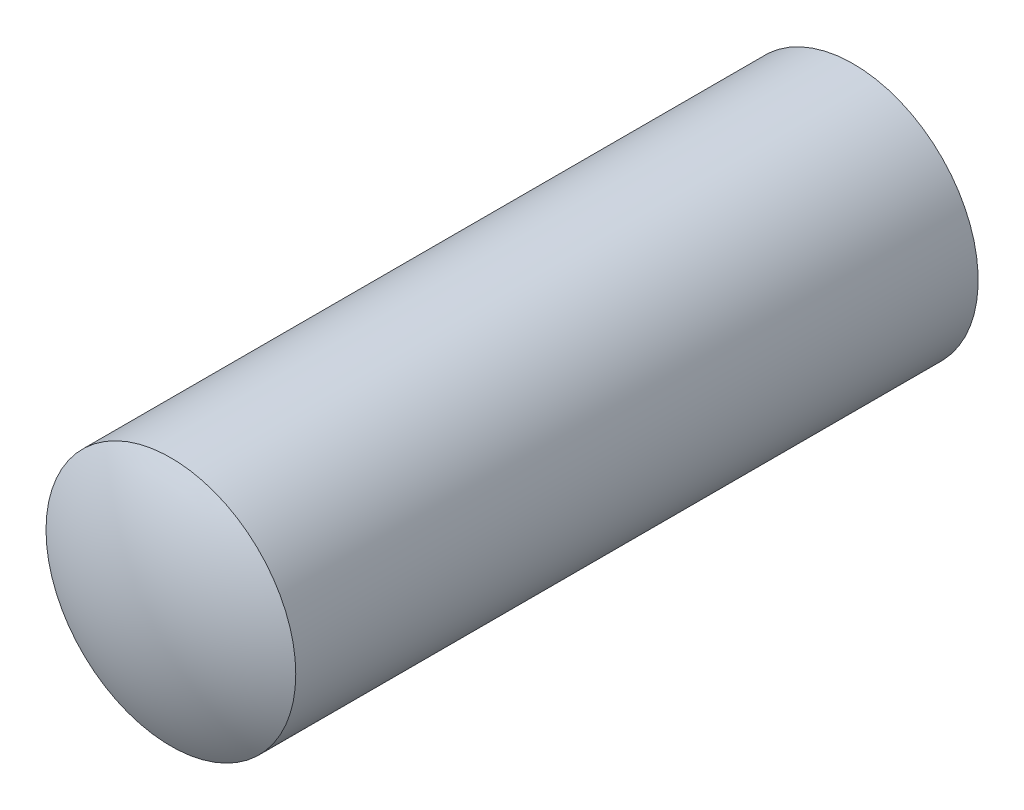
from build123d import *


with BuildPart() as part:
    # Logo3_bib1 → Revolve1 (revolve)
    with BuildSketch(Plane(origin=(0, 0, 0), x_dir=(-1, 0, 0), z_dir=(0, -1, 0))):
        with BuildLine():
            Line((0, 8), (0, -4))
            ThreePointArc((0, -4), (1.03527618, -3.863703305), (2, -3.464101615))
            Line((2, -3.464101615), (2, 7.464101615))
            ThreePointArc((2, 7.464101615), (1.03527618, 7.863703305), (0, 8))
        make_face()
    revolve(axis=Axis((0, 0, -47.537203702), (0, 0, 1)))


solid = part.part
